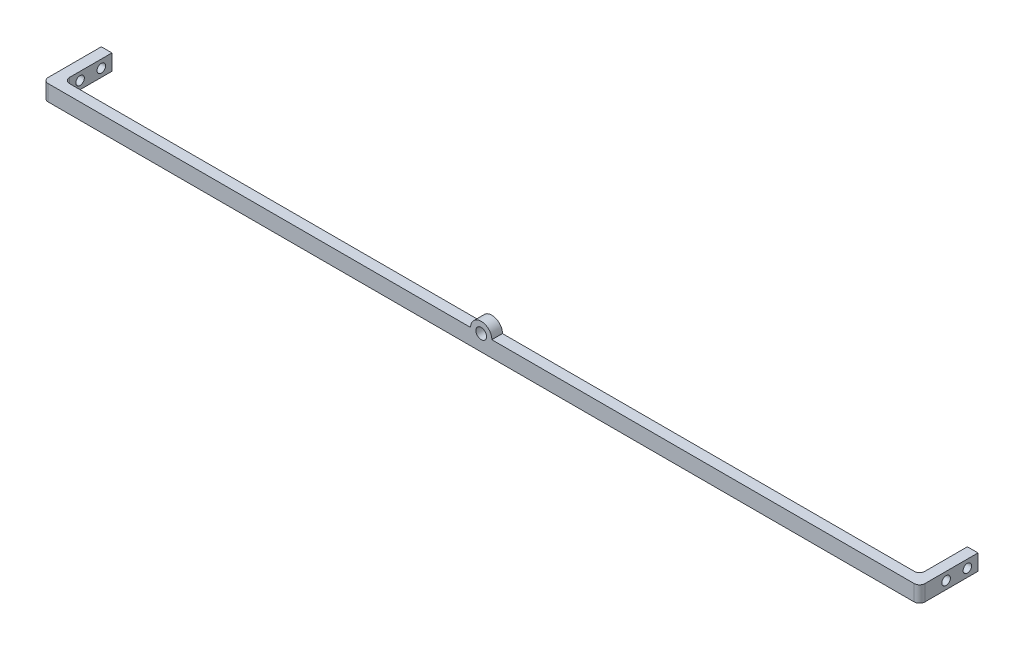
from build123d import *

# Parameters (mm, degrees)
SKETCH_1_R      = 5
EXTRUDE_1_DEPTH = 10
SKETCH_2_W      = 45
SKETCH_2_H      = 15
SKETCH_2_R      = 4
EXTRUDE_2_DEPTH = 10
EXTRUDE_START   = -10
SKETCH_3_W      = 45
SKETCH_3_H      = 15
SKETCH_3_R      = 4
EXTRUDE_3_DEPTH = 10
FILLET_1_R      = 5


with BuildPart() as part:
    # 草图1 → 凸台-拉伸1 (new body)
    with BuildSketch(Plane.XY):
        with BuildLine():
            Line((0, -15), (412.5, -15))
            Line((412.5, -15), (412.5, 0))
            Line((412.5, 0), (10, 0))
            ThreePointArc((10, 0), (0, 10), (-10, 0))
            Line((-10, 0), (-412.5, 0))
            Line((-412.5, 0), (-412.5, -15))
            Line((-412.5, -15), (0, -15))
        make_face()
        Circle(SKETCH_1_R, mode=Mode.SUBTRACT)
    extrude(amount=EXTRUDE_1_DEPTH)

    # 草图2 → 凸台-拉伸2 (add)
    with BuildSketch(Plane(origin=(412.5, 0, 0), x_dir=(0, 0, -1), z_dir=(1, 0, 0))):
        with Locations((22.5, -7.5)):
            Rectangle(SKETCH_2_W, SKETCH_2_H)
        with Locations((15, -7.5)):
            Circle(SKETCH_2_R, mode=Mode.SUBTRACT)
        with Locations((35, -7.5)):
            Circle(SKETCH_2_R, mode=Mode.SUBTRACT)
    extrude(amount=-EXTRUDE_2_DEPTH)

    # 草图3 → 凸台-拉伸3 (add)
    with BuildSketch(Plane.ZY.offset(412.5).offset(EXTRUDE_START)):
        with Locations((-22.5, -7.5)):
            Rectangle(SKETCH_3_W, SKETCH_3_H)
        with Locations(Location((-35, -7.5, 0), (0, 0, 180))):
            Circle(SKETCH_3_R, mode=Mode.SUBTRACT)
        with Locations(Location((-15, -7.5, 0), (0, 0, 180))):
            Circle(SKETCH_3_R, mode=Mode.SUBTRACT)
    extrude(amount=EXTRUDE_3_DEPTH)

    # 圆角1
    fillet_1_edges = [part.edges().sort_by_distance(p)[0] for p in [
        (-412.5, -7.5, 10),
        (402.5, -7.5, 0),
        (412.5, -7.5, 10),
        (-402.5, -7.5, 0),
    ]]
    fillet(fillet_1_edges, radius=FILLET_1_R)


solid = part.part
